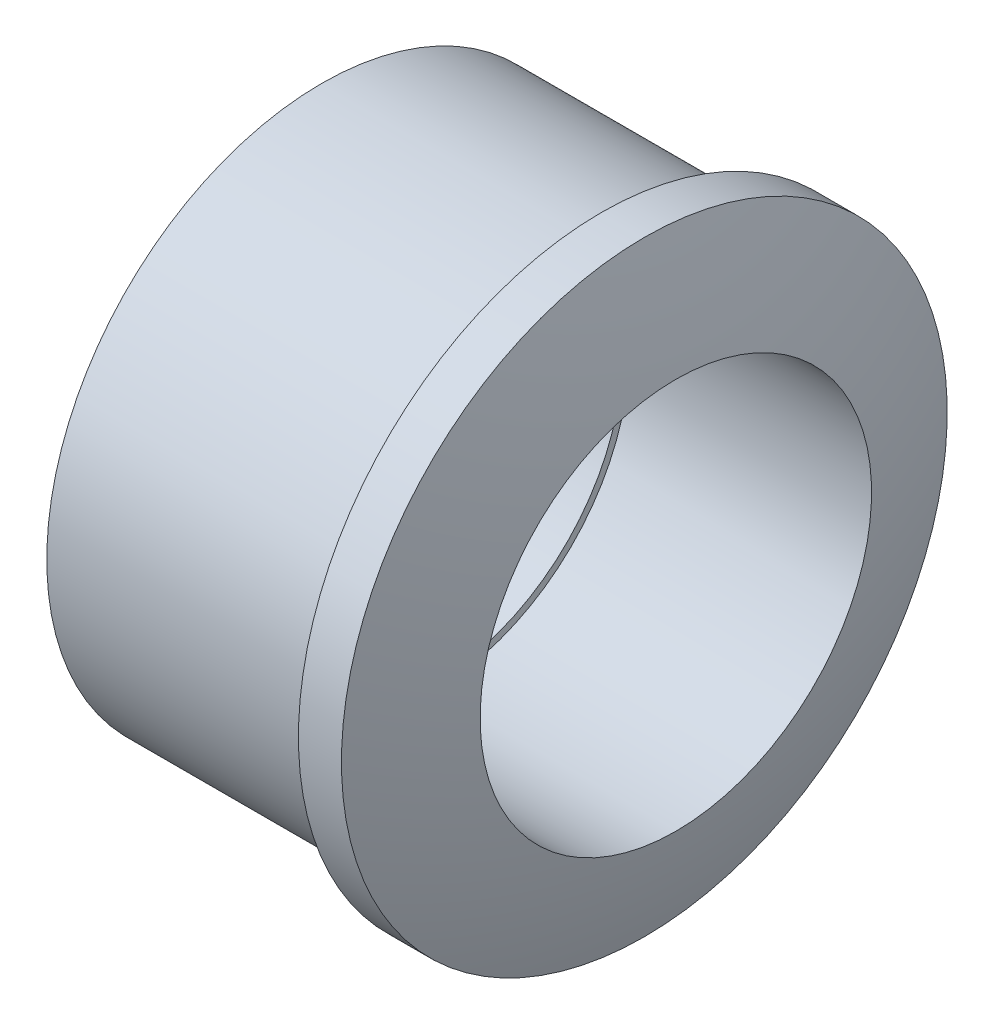
from build123d import *

# Parameters (mm, degrees)
SKETCH3_R          = 20.25
CUT_EXTRUDE2_DEPTH = 12
SKETCH4_R          = 21
CUT_EXTRUDE3_DEPTH = 53.80624963


with BuildPart() as part:
    # Sketch1 → Revolve1 (revolve)
    with BuildSketch(Plane.XY):
        with BuildLine():
            Line((0, 0), (0, 29.5))
            Line((0, 29.5), (30, 29.5))
            Line((30, 29.5), (30, 32.5))
            Line((30, 32.5), (34.617976782, 32.5))
            ThreePointArc((34.617976782, 32.5), (36.49055142, 26.803395685), (38, 21))
            Line((38, 21), (38, 0))
            Line((38, 0), (0, 0))
        make_face()
    revolve(axis=Axis((38, 0, 0), (-1, 0, 0)))

    # Sketch3 → Cut-Extrude2 (cut)
    with BuildSketch(Plane.ZY):
        with Locations(Location((0, 0, 0), (0, 0, 270))):
            Circle(SKETCH3_R)
    extrude(amount=-CUT_EXTRUDE2_DEPTH, mode=Mode.SUBTRACT)

    # Cut-Extrude1 cone 1 section (through the dimple's axis) → Cut-Extrude1 (revolve, cut)
    with BuildSketch(Plane.ZX):
        Polygon((0, 0), (29.5, 0), (0, 7.904501177), align=None)
    revolve(axis=Axis((0, 0, 0), (1, 0, 0)), mode=Mode.SUBTRACT)

    # Sketch4 → Cut-Extrude3 (cut, through all)
    with BuildSketch(Plane.ZY.offset(-12)):
        with Locations(Location((0, 0, 0), (0, 0, 270))):
            Circle(SKETCH4_R)
    extrude(amount=-CUT_EXTRUDE3_DEPTH, mode=Mode.SUBTRACT)


solid = part.part
